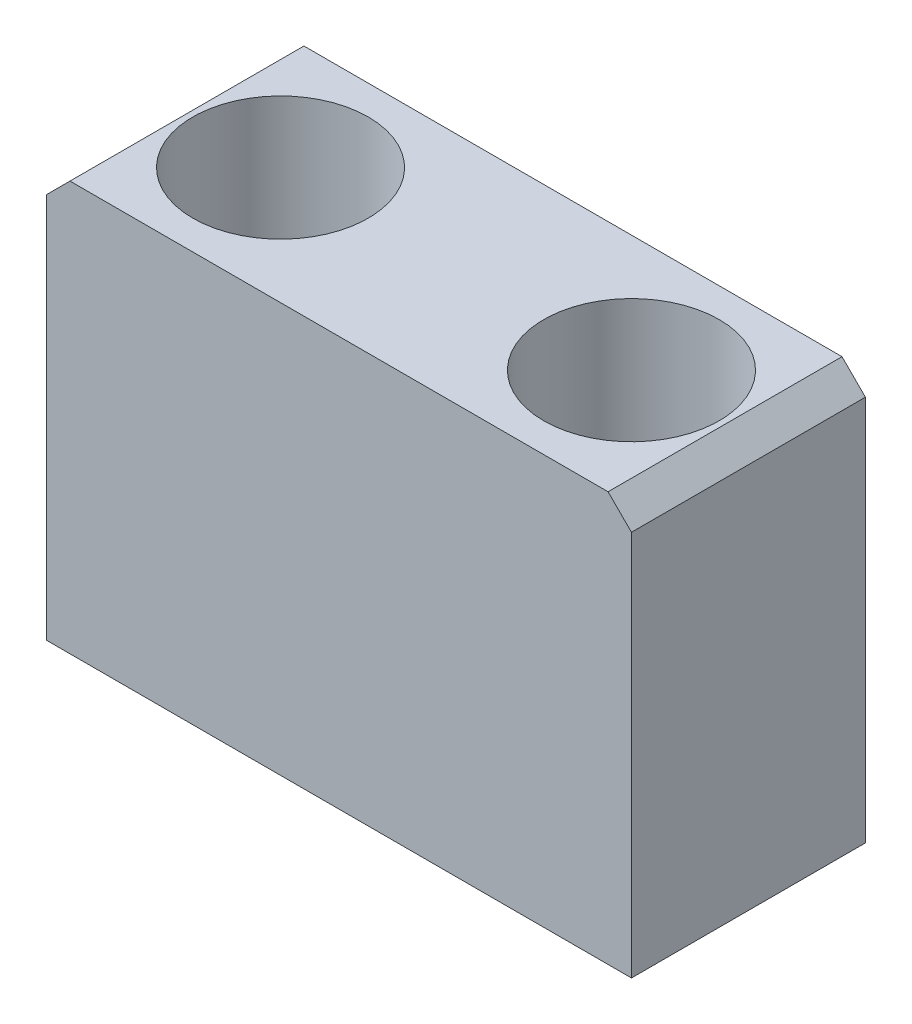
SolidWorks part; units mm, degrees
ref_plane "前视基准面" through (0, 0, 0) normal (0, 0, 1) x (1, 0, 0)
ref_plane "上视基准面" through (0, 0, 0) normal (0, 1, 0) x (1, 0, 0)
ref_plane "右视基准面" through (0, 0, 0) normal (1, 0, 0) x (0, 0, -1)
sketch "草图2" plane through (0, 0, 0) normal (0, 0, 1) x (1, 0, 0)
  line L1 (-25, 17.5) -> (25, 17.5)
  line L2 (-25, 17.5) -> (-25, -17.5)
  line L3 (-25, -17.5) -> (25, -17.5)
  line L4 (25, 17.5) -> (25, -17.5)
  line L5 (-25, 17.5) -> (25, -17.5) construction
  line L6 (-25, -17.5) -> (25, 17.5) construction
  point P0 (0, 0)
  dimension "D1" = 50
  dimension "D2" = 35
extrude "凸台-拉伸1" add sketch "草图2" along normal mid plane 20
hole_wizard "M8 六角凹头螺钉的柱形沉头孔1" positions "草图4" profile "草图5" counterbore size "M8" standard "ISO" end condition through all
sketch "草图4" plane through (0, 17.5, 0) normal (0, 1, 0) x (1, 0, 0)
  point P0 (15, 0)
  point P3 (-15, 0)
  dimension "D1" = 15
  dimension "D2" = 30
sketch "草图5" plane through (15, 17.5, 0) normal (1, 0, 0) x (0, 0, 1)
  line L0 (0, 0) -> (0, 35)
  line L1 (0, 35) -> (4.5, 35)
  line L3 (4.5, 35) -> (4.5, 15)
  line L4 (4.5, 15) -> (7.5, 15)
  line L5 (7.5, 15) -> (7.5, 0)
  line L7 (7.5, 0) -> (0, 0)
  line L11 (0, -6.35) -> (0, 107.95) construction
  dimension "通孔孔直径" = 9
  dimension "通孔孔深度" = 35
  dimension "柱形沉头孔直径" = 15
  dimension "柱形沉头孔深度" = 15
chamfer "倒角1" distance 2 angle 45 2 edges at (25, 17.5, 0) (-25, 17.5, 0)
